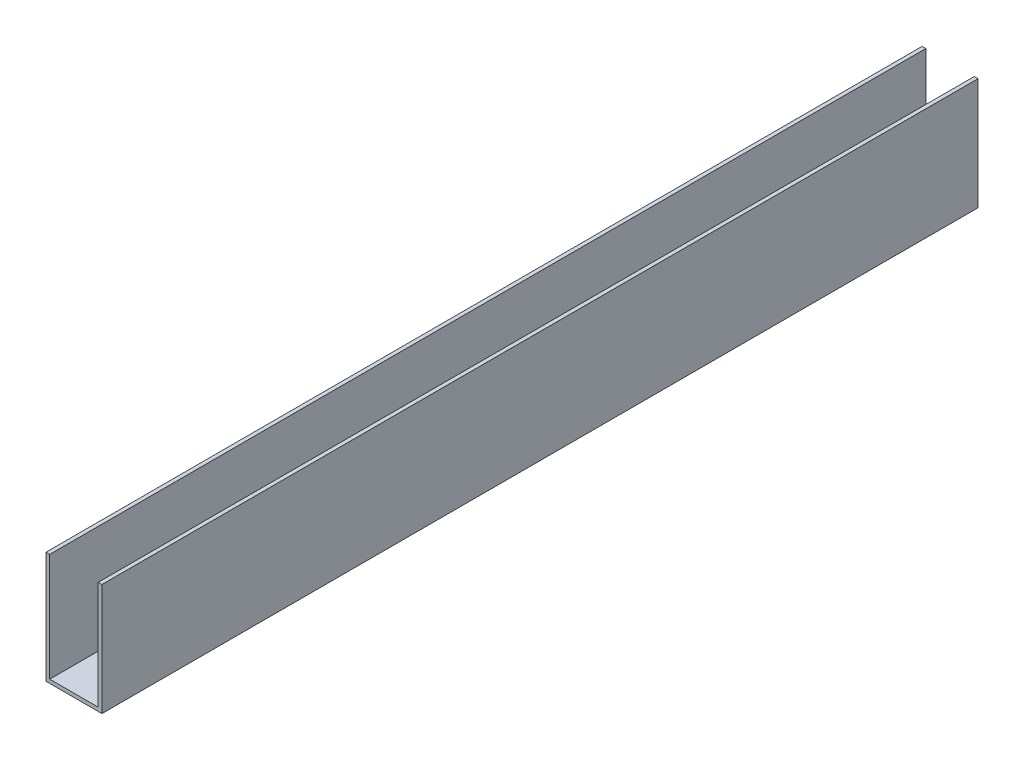
from build123d import *

# Parameters (mm, degrees)
SKETCH_1_W      = 30
SKETCH_1_H      = 60
EXTRUDE_1_DEPTH = 235
SHELL_1_T       = -2


with BuildPart() as part:
    # 草图1 → 凸台-拉伸1 (new, symmetric)
    with BuildSketch(Plane.XY):
        Rectangle(SKETCH_1_W, SKETCH_1_H)
    extrude(amount=EXTRUDE_1_DEPTH, both=True)

    # 抽壳1
    shell_1_openings = [part.faces().sort_by_distance(p)[0] for p in [
        (0, 0, 235),
        (0, 0, -235),
        (0, 30, 0),
    ]]
    offset(amount=SHELL_1_T, openings=shell_1_openings, kind=Kind.INTERSECTION)


solid = part.part
